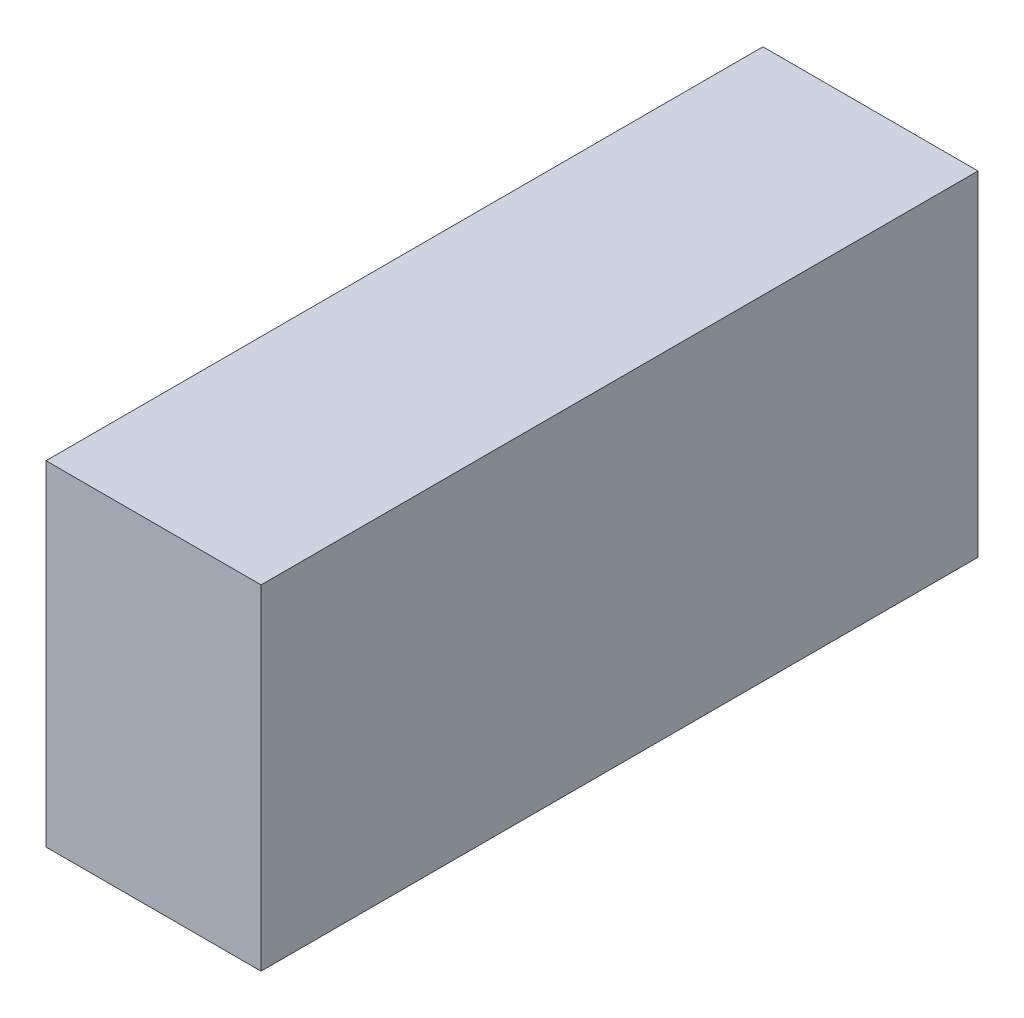
from build123d import *

# Parameters (mm, degrees)
SKETCH1_W           = 9
SKETCH1_H           = 30
BOSS_EXTRUDE1_DEPTH = 14


with BuildPart() as part:
    # Sketch1 → Boss-Extrude1 (new body)
    with BuildSketch(Plane(origin=(0, 0, 0), x_dir=(1, 0, 0), z_dir=(0, 1, 0))):
        Rectangle(SKETCH1_W, SKETCH1_H)
    extrude(amount=BOSS_EXTRUDE1_DEPTH)


solid = part.part
